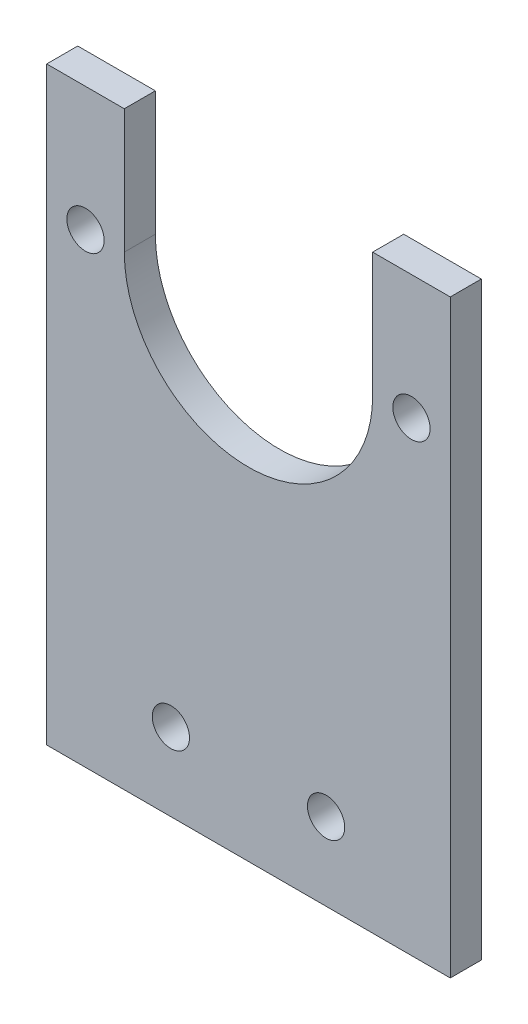
SolidWorks part; units mm, degrees
ref_plane "前视基准面" through (0, 0, 0) normal (0, 0, 1) x (1, 0, 0)
ref_plane "上视基准面" through (0, 0, 0) normal (0, 1, 0) x (1, 0, 0)
ref_plane "右视基准面" through (0, 0, 0) normal (1, 0, 0) x (0, 0, -1)
sketch "草图1" plane through (0, 0, 0) normal (0, 0, 1) x (1, 0, 0)
  line L0 (0, 0) -> (130, 0)
  line L1 (130, 0) -> (130, 190)
  line L2 (130, 190) -> (105, 190)
  line L3 (105, 190) -> (105, 150)
  line L5 (25, 150) -> (25, 190)
  line L6 (25, 190) -> (0, 190)
  line L7 (0, 190) -> (0, 0)
  line L8 (65, 213.3831) -> (65, -7.3328) construction
  arc A0 (25, 150) -> (105, 150) centre (65, 150) ccw
  circle A1 centre (117.5, 150) radius 6
  circle A2 centre (12.5, 150) radius 6
  circle A3 centre (40, 25) radius 6
  circle A4 centre (90, 25) radius 6
  dimension "D1" = 52.5
  dimension "D2" = 52.5
  dimension "D3" = 25
  dimension "D4" = 25
  dimension "D5" = 25
  dimension "D6" = 25
  dimension "D8" = 40
  dimension "D7" = 25
  dimension "D9" = 40
  dimension "D10" = 40
  dimension "D11" = 25
  dimension "D12" = 190
extrude "凸台-拉伸1" add sketch "草图1" along normal blind 10
